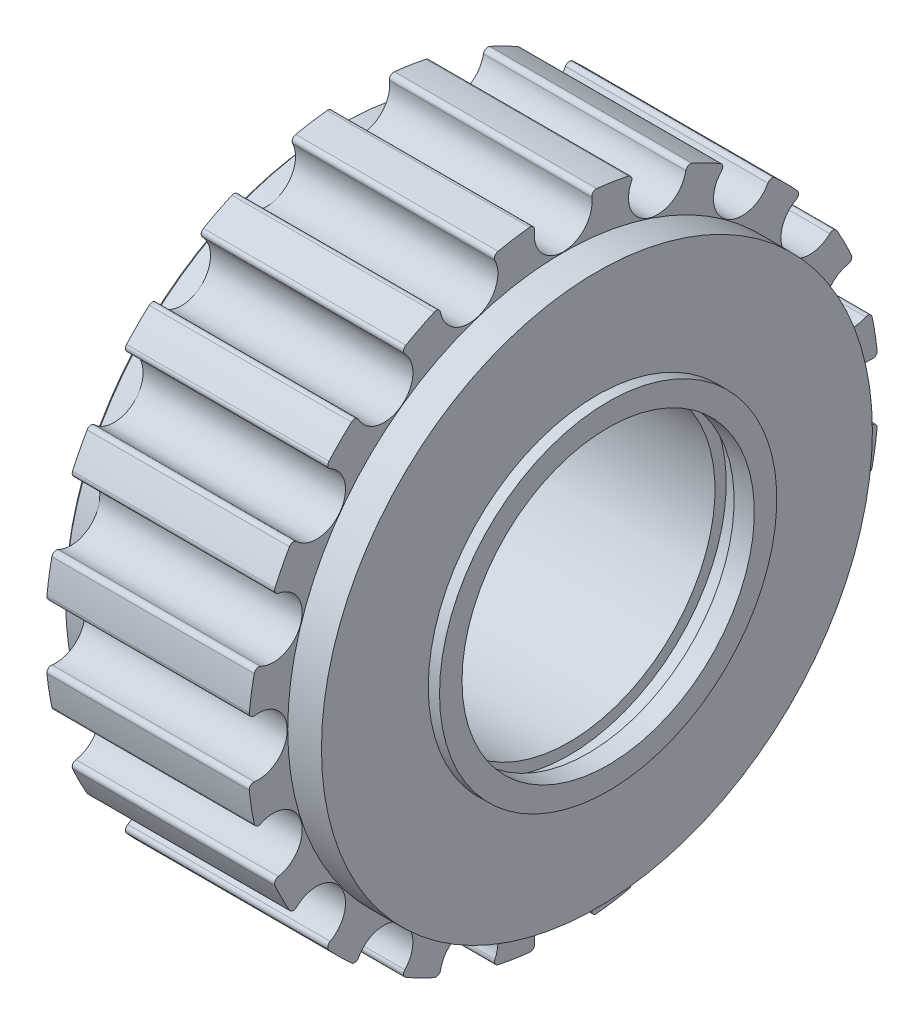
SolidWorks part; units mm, degrees
ref_plane "前视基准面" through (0, 0, 0) normal (0, 0, 1) x (1, 0, 0)
ref_plane "上视基准面" through (0, 0, 0) normal (0, 1, 0) x (1, 0, 0)
ref_plane "右视基准面" through (0, 0, 0) normal (1, 0, 0) x (0, 0, -1)
sketch "草图1" plane through (0, 0, 0) normal (0, 0, 1) x (1, 0, 0)
  line L0 (0, 0) -> (110.6379, 0) construction
  line L1 (0, 10.5) -> (4.5, 10.5)
  line L2 (4.5, 10.5) -> (4.5, 13)
  line L3 (4.5, 13) -> (20.5, 13)
  line L4 (20.5, 13) -> (20.5, 14)
  line L5 (20.5, 14) -> (22.2, 14)
  line L6 (22.2, 14) -> (22.2, 13)
  line L7 (22.2, 13) -> (24, 13)
  line L8 (24, 13) -> (24, 15)
  line L9 (24, 15) -> (23, 15)
  line L10 (23, 15) -> (23, 24.5)
  line L11 (23, 24.5) -> (20, 24.5)
  line L12 (20, 24.5) -> (20, 28.08)
  line L13 (20, 28.08) -> (2, 28.08)
  line L14 (2, 28.08) -> (2, 24.5)
  line L15 (2, 24.5) -> (0, 24.5)
  line L16 (0, 24.5) -> (0, 10.5)
  dimension "D1" = 4.5
  dimension "D2" = 2.5
  dimension "D3" = 16
  dimension "D4" = 1.7
  dimension "D5" = 1
  dimension "D6" = 1
  dimension "D7" = 1.8
  dimension "D8" = 2
  dimension "D9" = 1
  dimension "D10" = 9.5
  dimension "D11" = 3
  dimension "D12" = 3.58
  dimension "D13" = 18
  dimension "D14" = 3.58
  dimension "D15" = 2
  dimension "D16" = 10.5
revolve "旋转2" add sketch "草图1" angle 360 about L0
chamfer "倒角1" distance 0.25 angle 45 1 edges at (0, 0, 24.5)
sketch "草图2" plane through (20, 0, 0) normal (1, 0, 0) x (0, 0, -1)
  line L0 (0, 0) -> (0, 43.3766) construction
  circle A0 centre (0, 0) radius 28.08 construction
  arc A1 (2.9836, 27.921) -> (-2.9836, 27.921) centre (0, 0) ccw
  arc A2 (-2.545, 27.4676) -> (2.545, 27.4676) centre (0, 27.11) ccw
  arc A3 (-2.545, 27.4676) -> (-2.9836, 27.921) centre (-2.9411, 27.5233) ccw
  arc A4 (2.545, 27.4676) -> (2.9836, 27.921) centre (2.9411, 27.5233) cw
  point P7 (0, 28.08)
  point P8 (0, 24.54)
  dimension "D1" = 5.14
  dimension "D2" = 3.54
  dimension "D3" = 0.8
extrude "切除-拉伸1" cut sketch "草图2" against normal blind 18
pattern_circular "阵列(圆周)1" count 20 over 360 about axis through (0, 0, 0) along (1, 0, 0) of "切除-拉伸1"
